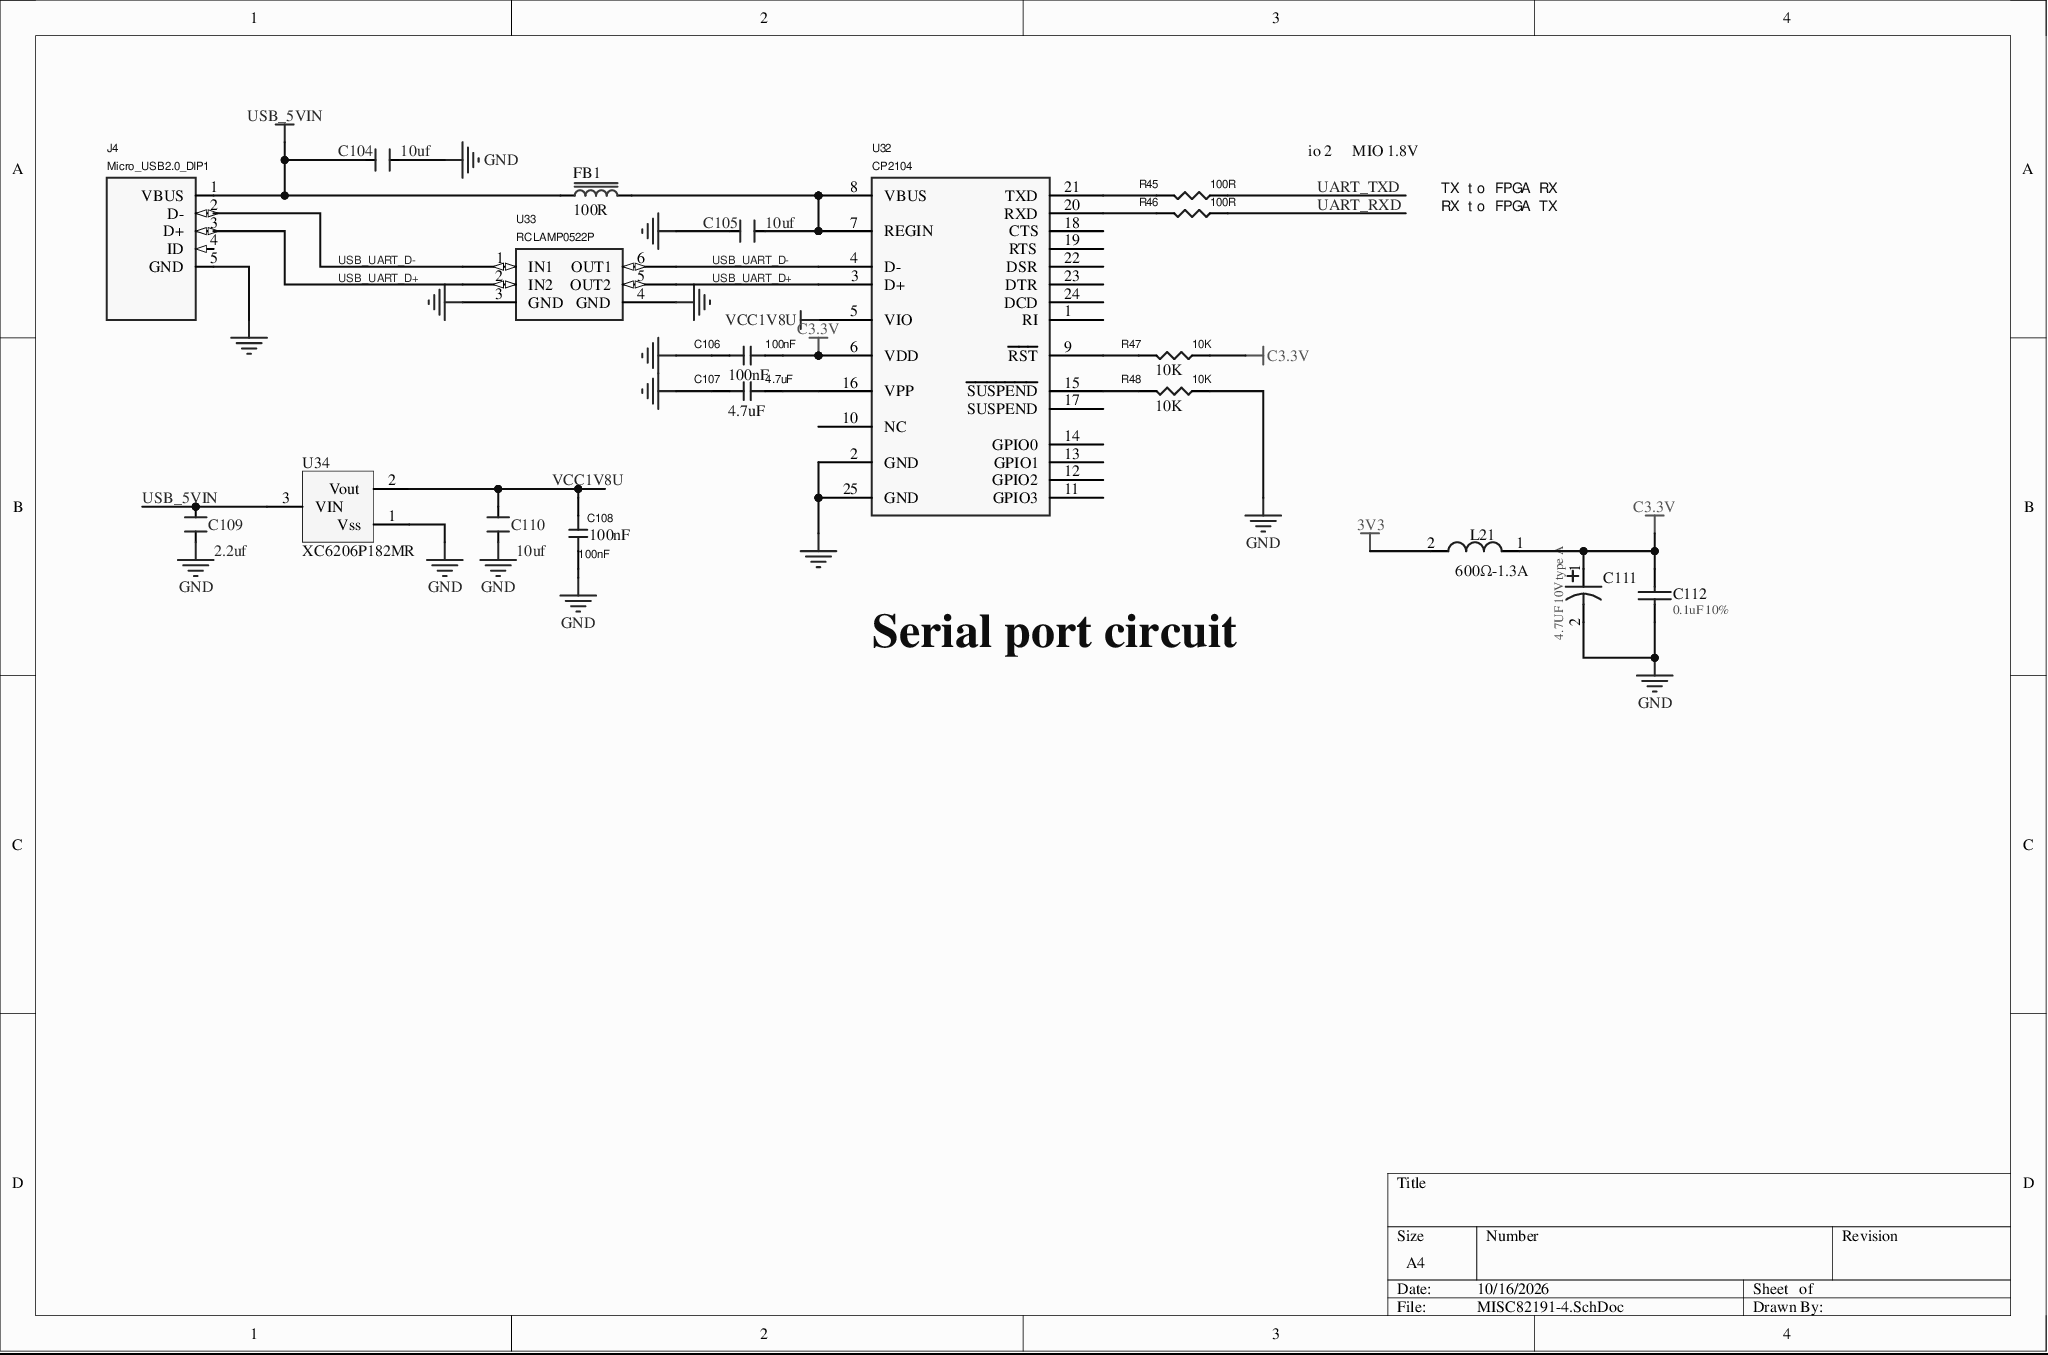
[diagram p0: MISC82191-4.SchDoc]
# Altium project MISC82191-2.PrjPcb (part 4 of 4)

## Sheet MISC82191-4.SchDoc
size A4

### Parts
C104  10uf  [0805]
C105  10uf  [0805]
C106  100nF  [0603]
C107  4.7uF  [0603]
C108  100nF  [0603]
C109  2.2uf  [0603]
C110  10uf  [0805]
C111  4.7UF 10V type A  [1005]
C112  0.1uF 10%  [0603]
FB1  100R  [0603]
J4  Micro_USB2.0_DIP1  [MINI-USB-TH_USB-MINI-2]
L21  600Ω-1.3A  [0603]
R45  100R  [0603]
R46  100R  [0603]
R47  10K  [0603]
R48  10K  [0603]
U32  CP2104  [QFN-24_L4.0-W4.0-P0.50-BL-EP2.7]
U33  RCLAMP0522P  [DFN-1610-6_L1.6-W1.0-P0.50-BL]
U34  XC6206P182MR  [SOT-23-3_L2.9-W1.6-P1.90-LS2.8-BR]

### Nets
3V3: L21.2
C3.3V: C106.2 C111.1 C112.1 L21.1 R47.2 U32.6(VDD)
GND: C104.1 C105.2 C106.1 C107.1 C108.1 C109.1 C110.1 C111.2 C112.2 J4.5(GND) R48.2 U32.2(GND) U32.25(GND) U33.3(GND) U33.4(GND) U34.1(Vss)  [project net DGND]
USB_5VIN: C104.2 C109.2 FB1.1 J4.1(VBUS) U34.3(VIN)
VCC1V8U: C108.2 C110.2 U32.5(VIO) U34.2(Vout)
UART_RXD: R46.2
UART_TXD: R45.2
USB_UART_D+: J4.3(D+) U32.3(D+) U33.2(IN2) U33.5(OUT2)
USB_UART_D-: J4.2(D-) U32.4(D-) U33.1(IN1) U33.6(OUT1)
NetC105_1: C105.1 FB1.2 U32.7(REGIN) U32.8(VBUS)
NetC107_2: C107.2 U32.16(VPP)
NetR45_1: R45.1 U32.21(TXD)
NetR46_1: R46.1 U32.20(RXD)
NetR47_1: R47.1 U32.9(~{RST})
NetR48_1: R48.1 U32.15(~{SUSPEND})

Not connected (* = marked no-connect by the designer): J4 4(ID)*; U32 1(RI) 10(NC) 11(GPIO3) 12(GPIO2) 13(GPIO1) 14(GPIO0) 17(SUSPEND) 18(CTS) 19(RTS) 22(DSR) 23(DTR) 24(DCD)

### Notes on the sheet
- io 2
- MIO 1.8V
- TX to FPGA RX
- RX to FPGA TX
- Serial port circuit

### Library data of the parts
C104 C105 C109 C110 = CAPACITOR: Generic Capacitor; DPN: *; Manufacturer: *
C106-C108 = CAP1: VC2: 0; MAX_TEMP: CTMAX; SLOPE: CSMAX; KNEE: CBMAX; CURRENT: CIMAX; VOLTAGE: CMAX; PSpiceTemplate: C^@REFDES %1 %2 ?TOLERANCE¦C^@REFDES¦ @VALUE ?IC/IC=@IC/ TC=@TC1,@TC2 ?TOLERANCE¦\n.model C^@REFDES CAP C=1 DEV=@TOLERANCE% TC1=@TC1 TC2=@TC2 VC1=@VC1 VC2=@VC2¦; DIST: FLAT; VC1: 0; TC1: 0; TC2: 0
  C106 C108: Value: 100nF
  C107: Value: 4.7uF
C111 = CAPACITOR
C112 = CAP: Capacitor
FB1 = Ferrite Bead: Generic Ferrite Bead; Value: 600; DPN: *; Manufacturer: *
J4 = Micro_USB2_0.0_DIP1
L21 = L: BLM18KG601SN-[0603]/Murata
R45-R48 = RES1: DIST: FLAT; PSpiceTemplate: R^@REFDES %1 %2 ?TOLERANCE¦R^@REFDES¦ @VALUE TC=@TC1,@TC2 ?TOLERANCE¦\n.model R^@REFDES RES R=1 DEV=@TOLERANCE% TC1=@TC1 TC2=@TC2¦; VOLTAGE: RVMAX; SLOPE: RSMAX; MAX_TEMP: RTMAX; POWER: RMAX; TC1: 0; TC2: 0
  R47 R48: Value: 10K
U34 = XC6206P332MR

## Nets that join several sheets
3V3: MISC82191-3 (28 pins), MISC82191-5 (C4.2 L4.3 U2.3), MISC82191-4 (L21.2)
13V: MISC82191-3 (25 pins), MISC82191-5 (5 pins)
-5.4V: MISC82191-3 (L104.3), MISC82191-5 (L9.3 TP4.1)
A6V: MISC82191-3 (L105.3), MISC82191-5 (C35.2 C36.2 C37.2 U6.3)
D5V: MISC82191-3 (39 pins), MISC82191-5 (7 pins)
DGND: MISC82191-3 (248 pins), MISC82191-5 (67 pins), MISC82191-4 (16 pins)
VCC1V8: MISC82191-3 (C88.2 U28.2 U28.10), MISC82191-5 (C3.1 U2.2)
UART_RXD: MISC82191-3 (P13.13), MISC82191-4 (R46.2)
UART_TXD: MISC82191-3 (P13.15), MISC82191-4 (R45.2)